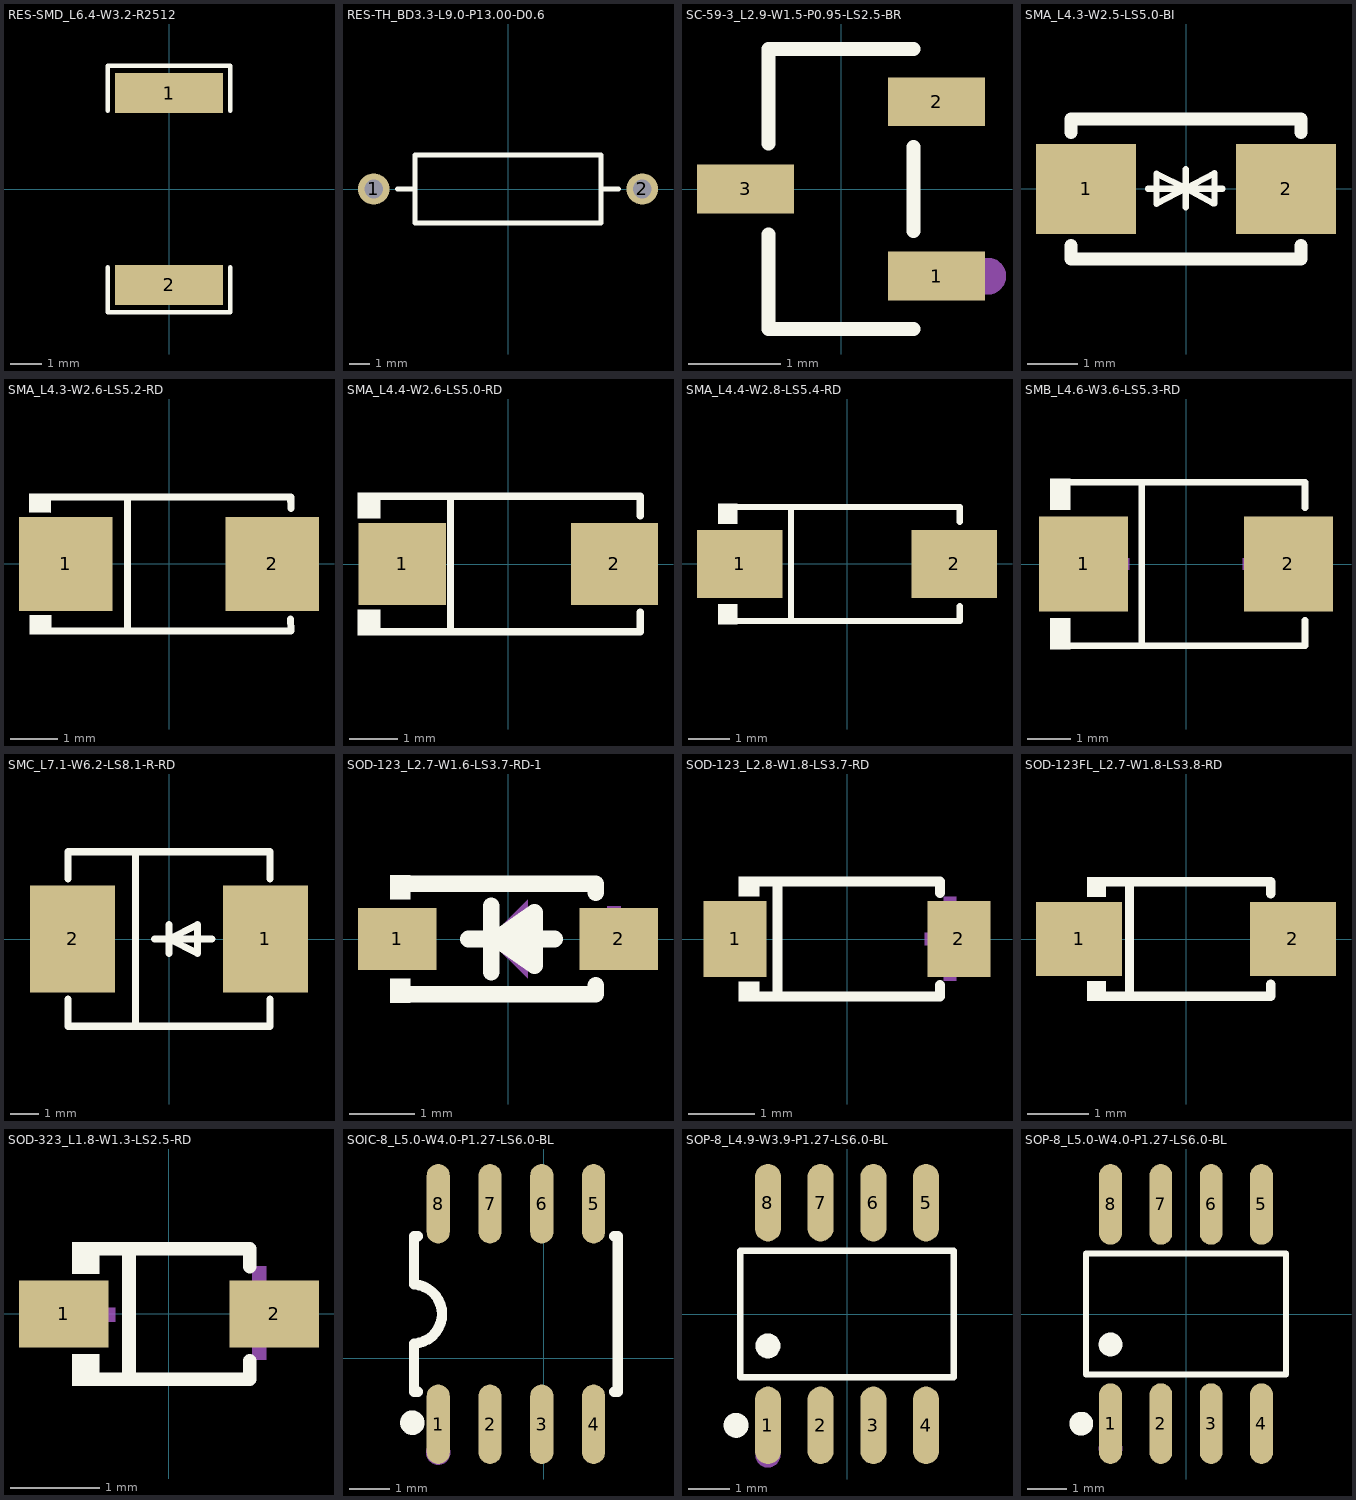
[diagram p0: the footprints below, top view; thin cyan lines are the x and y axes]
# Altium footprint library MISC84402-3.PcbLib: 74 footprints (part 4 of 5)
Each footprint in its own frame and in the unit in brackets; x right, y up, seen from the top. Pads: shape width x height; smd on the part's side, far side on the other; paste and mask are expansions set on the pad; w line width, h text height; cw(c..) or ccw(c..) is an arc to the next point about the centre after c.

## RES-SMD_L6.4-W3.2-R2512 [mm]
pads (2):
  rect 3.456x1.283 smd: 1(0,3.066) 2(0,-3.066)
Top Overlay:
  lines w0.152: -1.957,-2.501 -1.957,-3.936 1.957,-3.936 1.957,-2.501 ; -1.957,2.501 -1.957,3.936 1.957,3.936 1.957,2.501
Top Paste:
  region: -1.628,2.425 -0.688,2.425 -0.588,2.525 -0.588,2.761 -0.488,2.861 0.488,2.861 0.588,2.761 0.588,2.525 0.688,2.425 1.628,2.425 1.728,2.525 1.728,3.608 1.628,3.708 -1.628,3.708 -1.728,3.608 -1.728,2.525
  region: -1.628,-2.425 -0.688,-2.425 -0.588,-2.525 -0.588,-2.761 -0.488,-2.861 0.488,-2.861 0.588,-2.761 0.588,-2.525 0.688,-2.425 1.628,-2.425 1.728,-2.525 1.728,-3.608 1.628,-3.708 -1.628,-3.708 -1.728,-3.608 -1.728,-2.525

## RES-TH_BD3.3-L9.0-P13.00-D0.6 [mil]
pads (2):
  round 60 hole 36: 1(-255.91,0) 2(255.9,0)
Top Overlay:
  lines w10: -210,0 -180,0 ; 180,0 210,0 ; -177.16,-64.96 -177.16,64.96 177.16,64.96 177.16,-64.96 -177.16,-64.96

## SC-59-3_L2.9-W1.5-P0.95-LS2.5-BR [mm]
pads (3):
  rect 1.058x0.532 smd: 1(1.041,-0.95) 2(1.041,0.95) 3(-1.041,0)
Top Overlay:
  lines w0.152: -0.789,-0.495 -0.789,-1.526 0.789,-1.526 ; -0.789,0.495 -0.789,1.526 0.789,1.526 ; 0.789,-0.455 0.789,0.455
Mechanical 15:
  circle w0.2: c1.6,-0.95 r0.1

## SMA_L4.3-W2.5-LS5.0-BI [mm]
pads (2):
  rect 2x1.8 smd: 1(-2,0) 2(2,0)
Top Overlay:
  lines w0.127: -0.76,0.003 0.73,0.003 ; -0.59,-0.297 -0.59,0.303 -0.002,0.014 ; -0.576,-0.284 -0.004,0.015 ; -0.002,-0.367 -0.002,0.014 ; -0.002,0.395 -0.002,0.014 ; 0.54,-0.287 -0.002,0.014 ; 0.57,-0.287 0.57,0.313 -0.002,0.014
  lines w0.254: -2.3,-1.131 -2.3,-1.4 2.3,-1.4 2.3,-1.131 ; -2.3,1.131 -2.3,1.4 2.3,1.4 2.3,1.131

## SMA_L4.3-W2.6-LS5.2-RD [mm]
pads (2):
  rect 2x2 smd: 1(-2.2,0) 2(2.2,0)
Top Overlay:
  region: -2.512,-1.096 -2.513,-1.503 -2.973,-1.498 -2.969,-1.096
  region: -2.52,1.502 -2.521,1.096 -2.981,1.1 -2.977,1.502
  lines w0.152: -2.596,-1.426 2.596,-1.426 ; -2.596,1.426 2.596,1.426 2.603,1.187 ; -0.884,-1.426 -0.884,1.426 ; 2.593,-1.176 2.6,-1.415
Mechanical 15:
  region: 2.014,-0.675 2.014,0.675 1.811,0.675 1.811,-0.675
  region: 2.317,-0.101 2.317,0.101 1.507,0.101 1.507,-0.101
  region: -2.317,-0.101 -2.317,0.101 -1.507,0.101 -1.507,-0.101

## SMA_L4.4-W2.6-LS5.0-RD [mm]
pads (2):
  rect 1.8x1.7 smd: 1(-2.192,0) 2(2.192,0)
Top Overlay:
  region: -2.65,-1.477 -2.65,-0.949 -3.107,-0.949 -3.107,-1.477
  region: -2.65,1.477 -2.65,0.949 -3.107,0.949 -3.107,1.477
  lines w0.152: -2.726,-1.401 2.726,-1.401 2.726,-1 ; -2.726,1.401 2.726,1.401 2.726,1 ; -1.197,-1.401 -1.197,1.401
Mechanical 15:
  region: 2.153,-0.663 2.153,0.663 1.954,0.663 1.954,-0.663
  region: 2.451,-0.099 2.451,0.099 1.656,0.099 1.656,-0.099
  region: -2.451,-0.099 -2.451,0.099 -1.656,0.099 -1.656,-0.099

## SMA_L4.4-W2.8-LS5.4-RD [mm]
pads (2):
  rect 2.046x1.62 smd: 1(-2.566,0) 2(2.565,0)
Top Overlay:
  region: -2.625,1.44 -2.625,0.962 -3.082,0.962 -3.082,1.44
  region: -2.625,-1.44 -2.625,-0.962 -3.082,-0.962 -3.082,-1.44
  lines w0.152: -2.701,-1.364 2.701,-1.364 2.701,-1.013 ; -2.701,1.364 2.701,1.364 2.701,1.013 ; -1.339,-1.364 -1.339,1.364
Mechanical 15:
  region: -2.432,-0.097 -2.432,0.097 -1.659,0.097 -1.659,-0.097
  region: 2.432,-0.097 2.432,0.097 1.659,0.097 1.659,-0.097
  region: 2.142,-0.644 2.142,0.644 1.949,0.644 1.949,-0.644

## SMB_L4.6-W3.6-LS5.3-RD [mm]
pads (2):
  rect 2.047x2.192 smd: 1(-2.361,0) 2(2.361,0)
Top Overlay:
  region: -2.668,-1.962 -2.668,-1.249 -3.125,-1.249 -3.125,-1.962
  region: -2.668,1.962 -2.668,1.249 -3.125,1.249 -3.125,1.962
  lines w0.152: -2.744,-1.886 2.744,-1.886 2.744,-1.299 ; -2.744,1.886 2.744,1.886 2.744,1.299 ; -1.016,-1.886 -1.016,1.886
Mechanical 15:
  region: 1.989,-0.905 1.989,0.905 1.717,0.905 1.717,-0.905
  region: 2.396,-0.136 2.396,0.136 1.31,0.136 1.31,-0.136
  region: -2.396,-0.136 -2.396,0.136 -1.31,0.136 -1.31,-0.136

## SMC_L7.1-W6.2-LS8.1-R-RD [mm]
pads (2):
  rect 3.03x3.82 smd: 1(3.435,0) 2(-3.435,0)
Top Overlay:
  lines w0.254: -3.6,-2.141 -3.6,-3.11 3.6,-3.11 3.6,-2.141 ; -3.6,2.141 -3.6,3.11 3.6,3.11 3.6,2.141 ; -1.192,-3.11 -1.192,3.11 ; -0.508,0 1.524,0 ; 0,0.508 0,-0.508 0,0 ; 0,0 1.016,0.508 1.016,-0.508 0,0
Mechanical 15:
  region: -4.33,0.254 -2.552,0.254 -2.552,-0.254 -4.33,-0.254
  region: 3.181,-0.895 3.181,0.883 3.689,0.883 3.689,-0.895
  region: 2.54,0.254 4.318,0.254 4.318,-0.254 2.54,-0.254

## SOD-123_L2.7-W1.6-LS3.7-RD-1 [mm]
pads (2):
  rect 1.2x0.95 smd: 1(-1.7,0) 2(1.7,0)
Top Overlay:
  region: -1.502,-0.977 -1.502,-0.607 -1.806,-0.607 -1.806,-0.977
  region: -1.502,0.977 -1.502,0.607 -1.806,0.607 -1.806,0.977
  region: 0.406,-0.406 0.406,0.406 -0.178,0
  lines w0.254: -1.644,0.849 -1.643,0.85 -1.346,0.85 1.346,0.85 1.346,0.706 ; -1.639,-0.849 -1.638,-0.85 -1.346,-0.85 1.346,-0.85 1.346,-0.706 ; -0.61,0 -0.28,0 ; -0.254,-0.508 -0.254,0.508 ; 0.406,0 0.72,0 ; -0.178,0 0.406,-0.406 0.406,0.406 -0.178,0
Mechanical 15:
  region: -0.3,0 0.3,-0.6 0.3,0.6
  region: -2.042,0.124 -1.2,0.124 -1.2,-0.083 -2.042,-0.083
  region: 1.525,-0.338 1.525,0.504 1.732,0.504 1.732,-0.339
  region: 1.19,0.212 2.032,0.212 2.032,0.005 1.189,0.005

## SOD-123_L2.8-W1.8-LS3.7-RD [mm]
pads (2):
  rect 0.95x1.15 smd: 1(-1.693,0) 2(1.693,0)
Top Overlay:
  region: -1.33,-0.942 -1.33,-0.647 -1.635,-0.647 -1.635,-0.942
  region: -1.33,0.942 -1.33,0.647 -1.635,0.647 -1.635,0.942
  lines w0.152: -1.406,-0.866 1.406,-0.866 1.406,-0.698 ; -1.406,0.866 1.406,0.866 1.406,0.698 ; -1.049,-0.866 -1.049,0.866
Mechanical 15:
  region: 1.651,0.635 1.651,-0.629 1.461,-0.629 1.461,0.635
  region: 1.935,0.098 1.935,-0.092 1.177,-0.092 1.177,0.098
  region: -2.03,0.095 -2.03,-0.095 -1.272,-0.095 -1.272,0.095

## SOD-123FL_L2.7-W1.8-LS3.8-RD [mm]
pads (2):
  rect 1.4x1.2 smd: 1(-1.735,0) 2(1.735,0)
Top Overlay:
  region: -1.3,-1.002 -1.3,-0.682 -1.605,-0.682 -1.605,-1.002
  region: -1.3,1.002 -1.3,0.682 -1.605,0.682 -1.605,1.002
  lines w0.152: -1.376,-0.926 1.376,-0.926 1.376,-0.733 ; -1.376,0.926 1.376,0.926 1.376,0.733 ; -0.917,-0.876 -0.917,0.876
Mechanical 15:
  region: 1.747,-0.384 1.555,-0.384 1.555,0.384 1.747,0.384
  region: 2.035,0.096 2.035,-0.096 1.267,-0.096 1.267,0.096
  region: -2.032,0.127 -2.032,-0.065 -1.264,-0.065 -1.264,0.127

## SOD-323_L1.8-W1.3-LS2.5-RD [mm]
pads (2):
  rect 1x0.75 smd: 1(-1.173,0) 2(1.173,0)
Top Overlay:
  region: -0.775,-0.802 -0.775,-0.45 -1.08,-0.45 -1.08,-0.802
  region: -0.775,0.802 -0.775,0.45 -1.08,0.45 -1.08,0.802
  lines w0.152: -0.851,-0.726 0.901,-0.726 0.901,-0.52 ; -0.851,0.726 0.901,0.726 0.901,0.53 ; -0.447,-0.726 -0.447,0.726
Mechanical 15:
  region: 1.083,0.53 1.083,-0.51 0.927,-0.51 0.927,0.53
  region: 1.315,0.09 1.315,-0.066 0.691,-0.066 0.691,0.09
  region: -1.225,0.07 -1.225,-0.086 -0.601,-0.086 -0.601,0.07

## SOIC-8_L5.0-W4.0-P1.27-LS6.0-BL [mm]
pads (8):
  oval 0.568x1.95 smd: 1(-2.59,-1.623) 2(-1.32,-1.623) 3(-0.05,-1.623) 4(1.22,-1.623) 5(1.22,3.787) 6(-0.05,3.787) 7(-1.32,3.787) 8(-2.59,3.787)
Top Overlay:
  circle w0.3: c-3.225,-1.585 r0.15
  lines w0.254: -3.185,1.809 -3.185,2.582 -3.185,2.987 -3.094,2.987 ; -3.18,1.809 cw(c-3.225,1.082) -3.185,0.356 -3.185,-0.418 -3.185,-0.823 -3.094,-0.823 ; 1.723,-0.823 1.815,-0.823 1.815,-0.418 1.815,2.582 1.815,2.987 1.723,2.987
Mechanical 15:
  circle w0.3: c-2.59,-2.318 r0.15

## SOP-8_L4.9-W3.9-P1.27-LS6.0-BL [mm]
pads (8):
  oval 0.63x1.865 smd: 1(-1.905,-2.682) 2(-0.635,-2.682) 3(0.635,-2.682) 4(1.905,-2.682) 5(1.905,2.683) 6(0.635,2.683) 7(-0.635,2.683) 8(-1.905,2.683)
Top Overlay:
  circle w0.3: c-1.905,-0.769 r0.15
  circle w0.3: c-2.672,-2.682 r0.15
  lines w0.152: -2.576,-1.521 -2.576,1.521 2.576,1.521 2.576,-1.521 -2.576,-1.521
Mechanical 15:
  circle w0.3: c-1.905,-3.4 r0.15

## SOP-8_L5.0-W4.0-P1.27-LS6.0-BL [mm]
pads (8):
  oval 0.574x2.036 smd: 1(-1.905,-2.768) 2(-0.635,-2.768) 3(0.635,-2.768) 4(1.905,-2.768) 5(1.905,2.768) 6(0.635,2.768) 7(-0.635,2.768) 8(-1.905,2.768)
Top Overlay:
  circle w0.3: c-1.905,-0.769 r0.15
  circle w0.3: c-2.644,-2.768 r0.15
  lines w0.152: -2.526,-1.521 -2.526,1.521 2.526,1.521 2.526,-1.521 -2.526,-1.521
Mechanical 15:
  circle w0.3: c-1.905,-3.398 r0.15